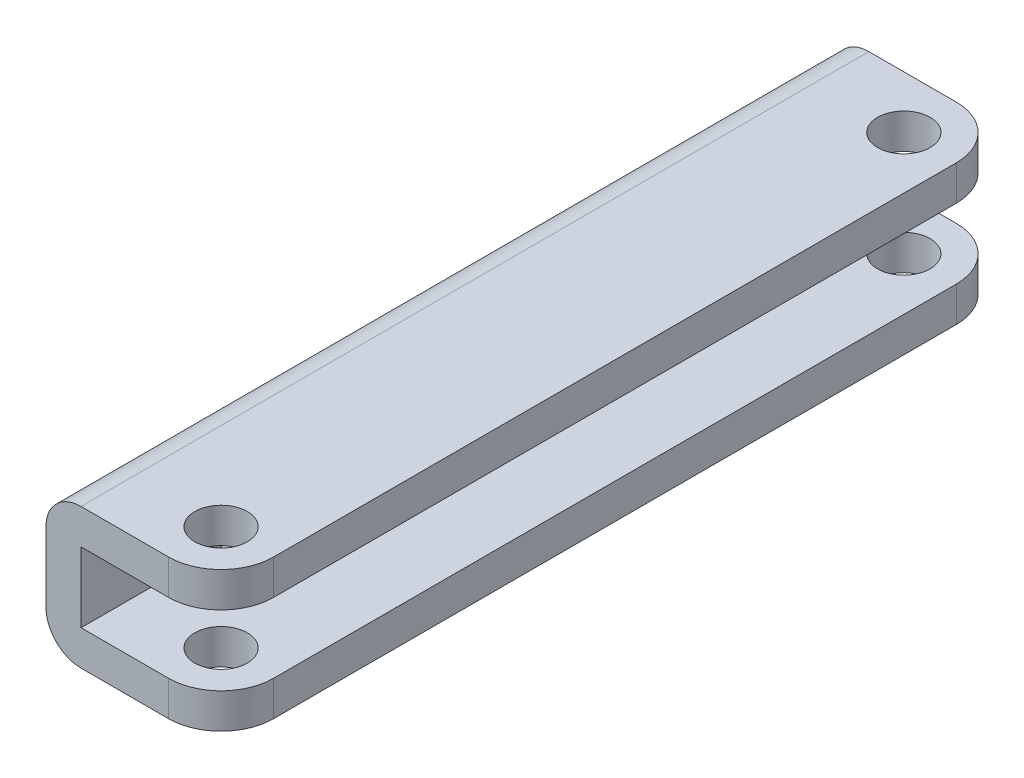
SolidWorks part; units mm, degrees
ref_plane "Front Plane" through (0, 0, 0) normal (0, 0, 1) x (1, 0, 0)
ref_plane "Top Plane" through (0, 0, 0) normal (0, 1, 0) x (1, 0, 0)
ref_plane "Right Plane" through (0, 0, 0) normal (1, 0, 0) x (0, 0, -1)
other "Configuration Table"
sketch "Sketch1" plane through (0, 0, 0) normal (0, 0, 1) x (1, 0, 0)
  line L0 (0, 4) -> (0, 2)
  line L1 (-8, 4) -> (0, 4)
  line L2 (-10, 2) -> (-10, -2)
  line L3 (-8, -4) -> (0, -4)
  line L5 (0, -4) -> (0, -2)
  line L7 (-8, 2) -> (0, 2)
  line L8 (-8, 2) -> (-8, -2)
  line L9 (-8, -2) -> (0, -2)
  arc A0 (-10, -2) -> (-8, -4) centre (-8, -2) ccw
  arc A1 (-8, 4) -> (-10, 2) centre (-8, 2) ccw
  point P0 (0, 0)
  point P6 (0, 0)
  point P14 (-10, -4)
  point P17 (-10, 4)
  dimension "D6" = 2
  dimension "D1" = 4
  dimension "D2" = 8
  dimension "D3" = 2
  dimension "D4" = 2
  dimension "D5" = 8
extrude "Boss-Extrude1" add sketch "Sketch1" along normal blind 45
sketch "Sketch2" plane through (0, -4, 0) normal (0, -1, 0) x (-1, 0, 0)
  line L0 (0, -45) -> (0, 0) construction
  line L1 (8, 0) -> (0, 0) construction
  line L2 (8, -45) -> (0, -45) construction
  circle A0 centre (3, -3) radius 1.5
  circle A1 centre (3, -42) radius 1.5
  dimension "D1" = 3
  dimension "D2" = 3
  dimension "D3" = 3
  dimension "D4" = 3
  dimension "D5" = 3
  dimension "D6" = 3
extrude "Cut-Extrude1" cut sketch "Sketch2" against normal through all
fillet "Fillet1" radius 3 4 edges at (0, -3, 0) (0, 3, 0) (0, 3, 45) (0, -3, 45)
